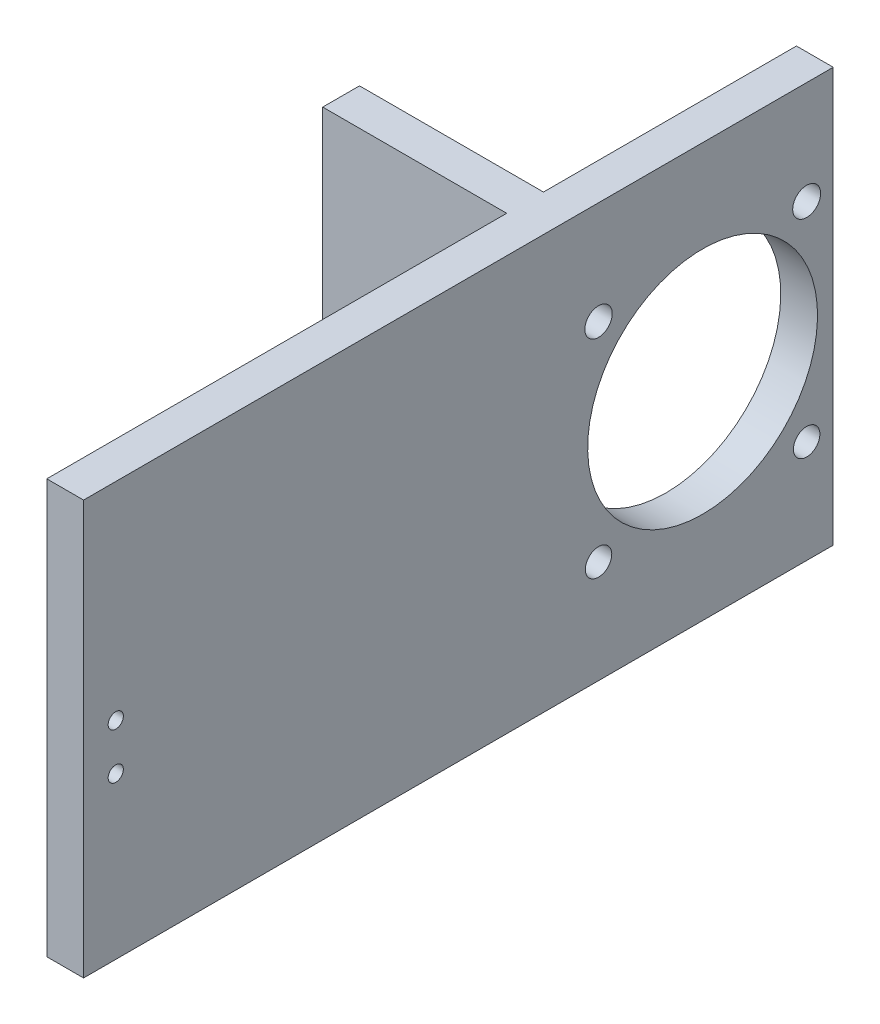
SolidWorks part; units mm, degrees
ref_plane "Front Plane" through (0, 0, 0) normal (0, 0, 1) x (1, 0, 0)
ref_plane "Top Plane" through (0, 0, 0) normal (0, 1, 0) x (1, 0, 0)
ref_plane "Right Plane" through (0, 0, 0) normal (1, 0, 0) x (0, 0, -1)
sketch "Sketch1" plane through (0, 0, 0) normal (0, 0, 1) x (1, 0, 0)
  line L1 (-60, 45) -> (60, 45)
  line L2 (-60, 45) -> (-60, -45)
  line L3 (-60, -45) -> (60, -45)
  line L4 (60, 45) -> (60, -45)
  line L5 (-60, 45) -> (60, -45) construction
  line L6 (-60, -45) -> (60, 45) construction
  circle A0 centre (0, 0) radius 40
  point P0 (0, 0)
  dimension "D3" = 80
  dimension "D1" = 120
  dimension "D2" = 90
extrude "Boss-Extrude1" add sketch "Sketch1" along normal blind 8
sketch "Sketch3" plane through (-60, 0, 0) normal (-1, 0, 0) x (0, 0, 1)
  line L4 (0, 45) -> (0, -45)
  line L5 (0, -45) -> (8, -45)
  line L6 (8, -45) -> (8, 45)
  line L7 (8, 45) -> (0, 45)
  line L8 (0, 45) -> (0, -45)
  line L9 (0, -45) -> (8, -45)
  line L10 (8, -45) -> (8, 45)
  line L11 (8, 45) -> (0, 45)
  dimension "D1" = 0
extrude "Boss-Extrude2" add sketch "Sketch3" along normal blind 50
sketch "Sketch4" plane through (0, 0, 8) normal (0, 0, 1) x (1, 0, 0)
  line L0 (60, 45) -> (-110, 45) construction
  line L1 (-70, 45) -> (-62, 45)
  line L2 (-70, 45) -> (-70, -45)
  line L3 (-70, -45) -> (-62, -45)
  line L4 (-62, 45) -> (-62, -45)
  line L5 (-110, -45) -> (60, -45) construction
  line L6 (-110, -45) -> (-110, 45) construction
  dimension "D1" = 8
  dimension "D2" = 40
extrude "Boss-Extrude3" add sketch "Sketch4" along normal blind 100
sketch "Sketch5" plane through (0, 0, 8) normal (0, 0, 1) x (1, 0, 0)
  line L1 (-62, 45) -> (116.6848, 45)
  line L2 (-62, 45) -> (-62, -103.4325)
  line L3 (-62, -103.4325) -> (116.6848, -103.4325)
  line L4 (116.6848, 45) -> (116.6848, -103.4325)
extrude "Cut-Extrude1" cut sketch "Sketch5" against normal through all
sketch "Sketch6" plane through (0, 0, 0) normal (0, 0, -1) x (-1, 0, 0)
  line L4 (70, -45) -> (70, 45)
  line L5 (62, -45) -> (70, -45)
  line L6 (62, 45) -> (62, -45)
  line L7 (70, 45) -> (62, 45)
  line L8 (70, -45) -> (70, 45)
  line L9 (62, -45) -> (70, -45)
  line L10 (62, 45) -> (62, -45)
  line L11 (70, 45) -> (62, 45)
  dimension "D1" = 0
extrude "Boss-Extrude4" add sketch "Sketch6" along normal blind 55
sketch "Sketch7" plane through (-70, 0, 0) normal (-1, 0, 0) x (0, 0, 1)
  circle A1 centre (-49.2274, 22.6274) radius 3.0364
  circle A2 centre (-49.2274, -22.6274) radius 2.8739
  circle A3 centre (-3.9726, -22.6274) radius 2.8744
  circle A4 centre (-3.9726, 22.6274) radius 2.9814
  circle A5 centre (-26.6, 0.0091) radius 24.9909
extrude "Cut-Extrude2" cut sketch "Sketch7" against normal blind 35
hole_wizard "M4 Tapped Hole1" positions "Sketch8" profile "Sketch9" tap size "M4" standard "GB"
sketch "Sketch8" plane through (-70, 0, 0) normal (-1, 0, 0) x (0, 0, 1)
  point P0 (101, 0)
  point P3 (101, -10)
sketch "Sketch9" plane through (-70, 0, 101) normal (0, 1, 0) x (0, 0, 1)
  line L0 (0, 0) -> (0, 11.0914)
  line L1 (0, 11.0914) -> (1.65, 10.1)
  line L2 (1.65, 10.1) -> (1.65, 0)
  line L5 (1.65, 0) -> (0, 0)
  line L10 (0, 11.0914) -> (-1.65, 10.1) construction
  line L11 (0, -6.35) -> (0, 107.95) construction
  dimension "螺纹孔钻头直径" = 3.3
  dimension "螺纹孔钻头深度" = 10.1
  dimension "导头角度" = 118
cosmetic thread "Cosmetic Thread1" parameters "D1"=8, "D2"=4
cosmetic thread "Cosmetic Thread2" parameters "D1"=8, "D2"=4
